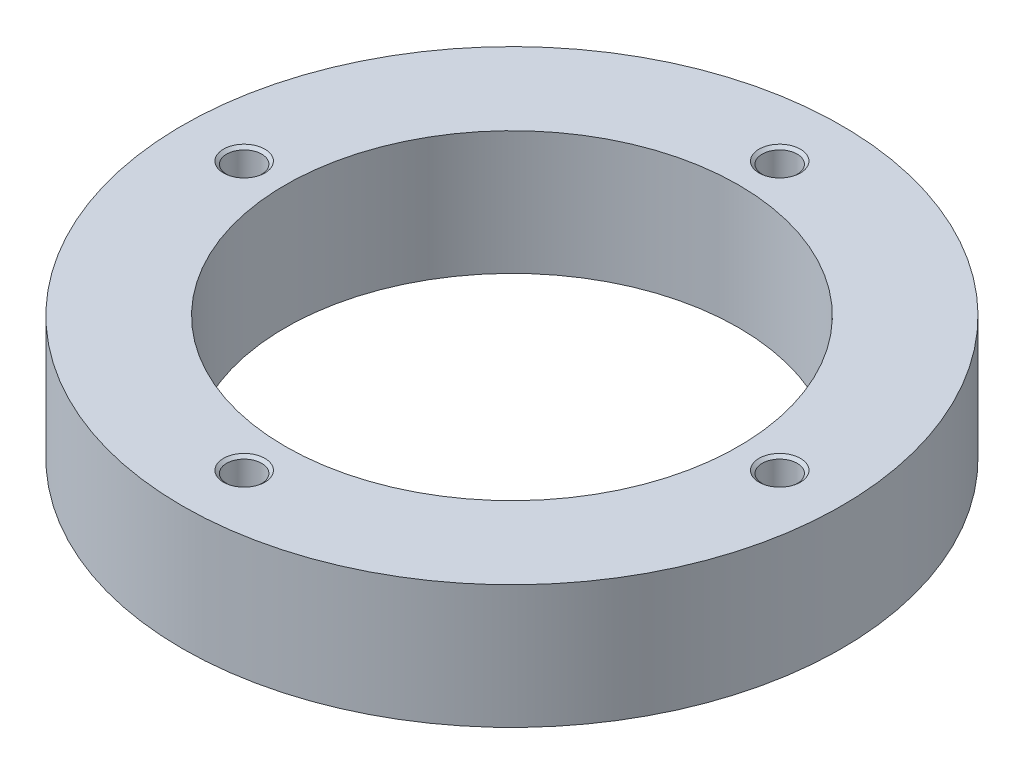
from build123d import *

# Parameters (mm, degrees)
SKETCH1_R                    = 80
SKETCH1_R_2                  = 55
BOSS_EXTRUDE1_DEPTH          = 30
M10_TAPPED_HOLE1_D           = 8.5
M10_TAPPED_HOLE1_DEPTH       = 22
M10_TAPPED_HOLE1_CSINK_D     = 10.05
M10_TAPPED_HOLE1_CSINK_ANGLE = 100
M10_TAPPED_HOLE1_TIP         = 2.553657631


with BuildPart() as part:
    # Sketch1 → Boss-Extrude1 (new body)
    with BuildSketch(Plane(origin=(0, 0, 0), x_dir=(1, 0, 0), z_dir=(0, 1, 0))):
        with Locations(Location((0, 0, 0), (0, 0, 270))):
            Circle(SKETCH1_R)
        with Locations(Location((0, 0, 0), (0, 0, 270))):
            Circle(SKETCH1_R_2, mode=Mode.SUBTRACT)
    extrude(amount=BOSS_EXTRUDE1_DEPTH)

    # M10 Tapped Hole1
    with Locations(Plane(origin=(0, 30, 0), x_dir=(1, 0, 0), z_dir=(0, 1, 0))):
        with Locations((0, 65), (65, 0), (0, -65), (-65, 0)):
            CounterSinkHole(M10_TAPPED_HOLE1_D / 2, M10_TAPPED_HOLE1_CSINK_D / 2, depth=M10_TAPPED_HOLE1_DEPTH, counter_sink_angle=M10_TAPPED_HOLE1_CSINK_ANGLE)
            with Locations((0, 0, -(M10_TAPPED_HOLE1_DEPTH + M10_TAPPED_HOLE1_TIP / 2))):  # 118° drill point
                Cone(0, M10_TAPPED_HOLE1_D / 2, M10_TAPPED_HOLE1_TIP, mode=Mode.SUBTRACT)


solid = part.part
